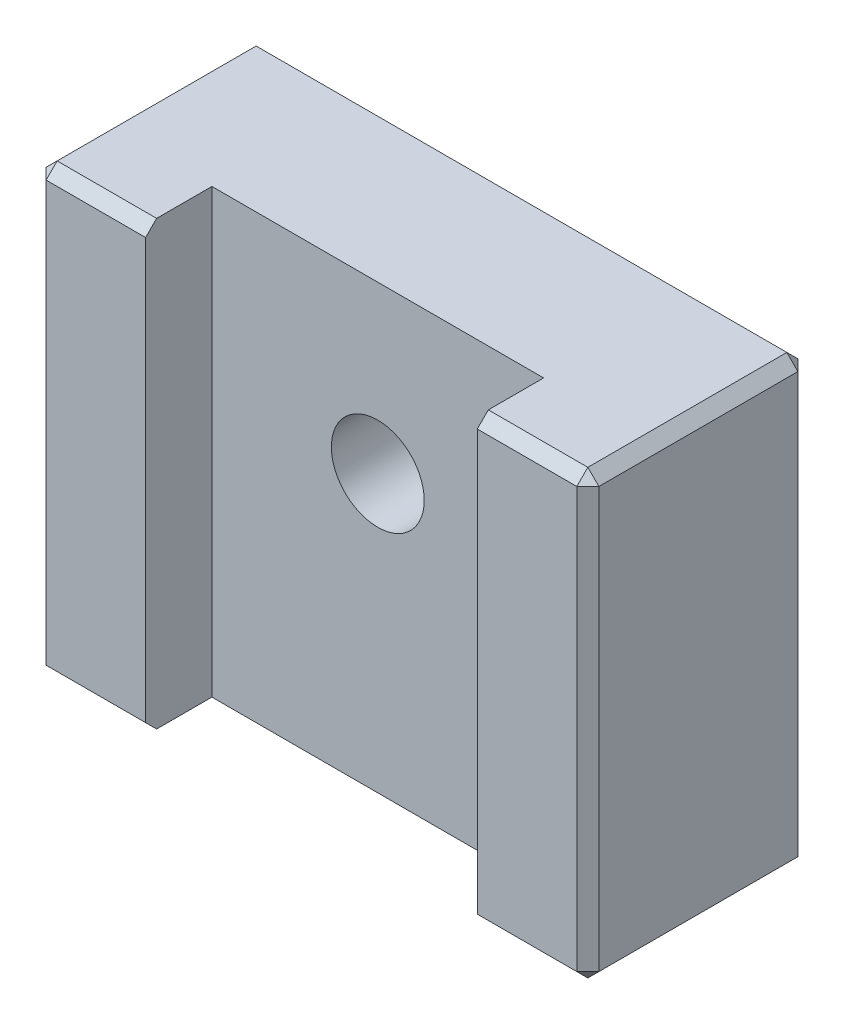
SolidWorks part; units mm, degrees
material "A6061"
ref_plane "Front Plane" through (0, 0, 0) normal (0, 0, 1) x (1, 0, 0)
ref_plane "Top Plane" through (0, 0, 0) normal (0, 1, 0) x (1, 0, 0)
ref_plane "Right Plane" through (0, 0, 0) normal (1, 0, 0) x (0, 0, -1)
sketch "Sketch1" plane through (0, 0, 0) normal (0, 0, 1) x (1, 0, 0)
  line L1 (-12.5, -10) -> (12.5, -10)
  line L2 (-12.5, -10) -> (-12.5, 10)
  line L3 (-12.5, 10) -> (12.5, 10)
  line L4 (12.5, -10) -> (12.5, 10)
  line L5 (-12.5, -10) -> (12.5, 10) construction
  line L6 (-12.5, 10) -> (12.5, -10) construction
  point P0 (0, 0)
  dimension "D1" = 25
  dimension "D2" = 20
extrude "Boss-Extrude1" add sketch "Sketch1" along normal blind 10
sketch "Sketch2" plane through (0, 0, 10) normal (0, 0, 1) x (1, 0, 0)
  line L0 (-12.5, -10) -> (12.5, -10) construction
  line L1 (-7.5, 10) -> (7.5, 10)
  line L2 (-7.5, 10) -> (-7.5, -10)
  line L3 (-7.5, -10) -> (7.5, -10)
  line L4 (7.5, 10) -> (7.5, -10)
  line L5 (-7.5, 10) -> (7.5, -10) construction
  line L6 (-7.5, -10) -> (7.5, 10) construction
  point P0 (0, 0)
  dimension "D1" = 15
extrude "Cut-Extrude1" cut sketch "Sketch2" against normal blind 3
hole_wizard "M5 Tapped Hole1" positions "Sketch4" profile "Sketch3" tap size "M5" standard "GB" end condition through all
sketch "Sketch4" plane through (0, 0, 7) normal (0, 0, 1) x (1, 0, 0)
  line L0 (7.5, 10) -> (-7.5, 10) construction
  point P0 (0, 2.5)
  dimension "D1" = 7.5
cosmetic thread "Cosmetic Thread1" parameters "D2"=5
sketch "Sketch3" plane through (0, 2.5, 7) normal (1, 0, 0) x (0, -1, 0)
  line L0 (0, 0) -> (0, 7)
  line L1 (0, 7) -> (2.1, 7)
  line L2 (2.1, 7) -> (2.1, 0)
  line L5 (2.1, 0) -> (0, 0)
  line L11 (0, -6.35) -> (0, 107.95) construction
  dimension "通孔螺纹孔钻头直径" = 4.2
  dimension "通孔螺纹孔钻头深度" = 7
hole_wizard "M5 Tapped Hole2" positions "Sketch6" profile "Sketch5" tap size "M5" standard "GB"
sketch "Sketch6" plane through (0, -10, 0) normal (0, -1, 0) x (-1, 0, 0)
  line L0 (-8.5, -4) -> (8.5, -4)
  line L2 (12.5, 0) -> (-12.5, 0) construction
  line L3 (-12.5, -10) -> (-12.5, 0) construction
  line L4 (12.5, -10) -> (12.5, 0) construction
  point P0 (8.5, -4)
  point P2 (-8.5, -4)
  dimension "D1" = 4
  dimension "D2" = 4
  dimension "D3" = 4
sketch "Sketch5" plane through (-8.5, -10, 4) normal (1, 0, 0) x (0, 0, -1)
  line L0 (0, 0) -> (0, 13.6618)
  line L1 (0, 13.6618) -> (2.1, 12.4)
  line L2 (2.1, 12.4) -> (2.1, 0)
  line L5 (2.1, 0) -> (0, 0)
  line L10 (0, 13.6618) -> (-2.1, 12.4) construction
  line L11 (0, -6.35) -> (0, 107.95) construction
  dimension "螺纹孔钻头直径" = 4.2
  dimension "螺纹孔钻头深度" = 12.4
  dimension "导头角度" = 118
cosmetic thread "Cosmetic Thread2" parameters "D1"=10, "D2"=5
cosmetic thread "Cosmetic Thread3" parameters "D1"=10, "D2"=5
chamfer "Chamfer1" distance 0.5 angle 45 14 edges at (10, -10, 10) (-10, -10, 10) (10, 10, 10) (-10, 10, 10) (12.5, 0, 10) (12.5, -10, 5) (12.5, 10, 5) (12.5, 0, 0) (0, 10, 0) (0, -10, 0) (-12.5, -10, 5) (-12.5, 0, 0) (-12.5, 10, 5) (-12.5, 0, 10)
